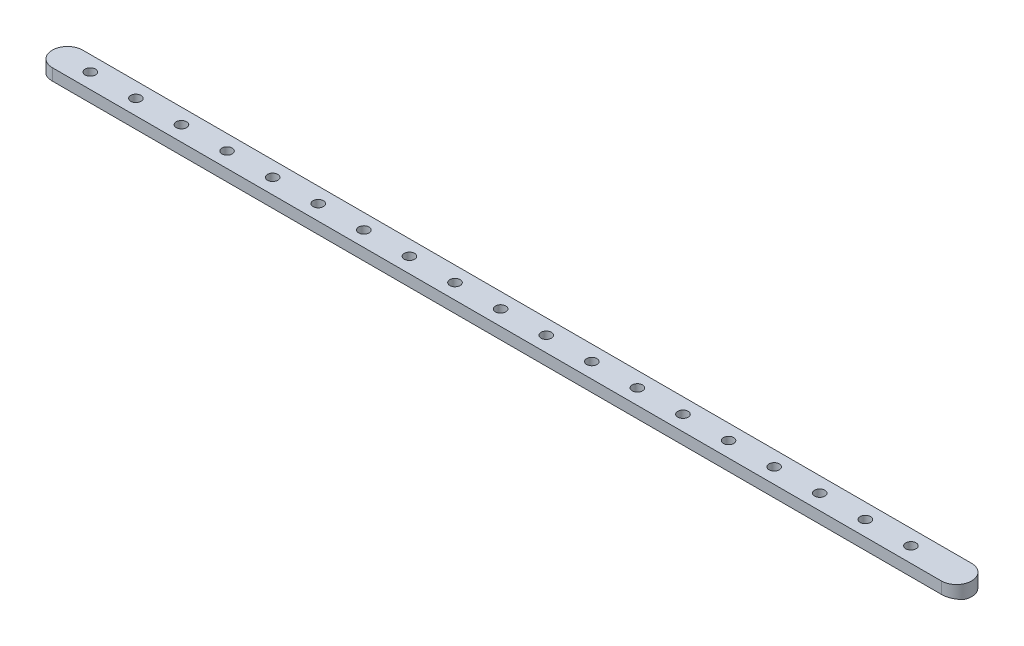
from build123d import *

# Parameters (mm, degrees)
BOSS_EXTRUDE1_DEPTH = 9
M8_TAPPED_HOLE1_D   = 6.8
LPATTERN1_COUNT     = 19
LPATTERN1_PITCH     = 30
CUT_EXTRUDE1_START  = -200
CUT_EXTRUDE1_DEPTH  = 705.20277905


with BuildPart() as part:
    # Sketch1 → Boss-Extrude1 (new body)
    with BuildSketch(Plane(origin=(0, 0, 0), x_dir=(1, 0, 0), z_dir=(0, 1, 0))):
        with BuildLine():
            Line((-90.976744186, 10), (494.023255814, 10))
            ThreePointArc((494.023255814, 10), (504.023255814, 0), (494.023255814, -10))
            Line((494.023255814, -10), (-90.976744186, -10))
            ThreePointArc((-90.976744186, -10), (-100.976744186, 0), (-90.976744186, 10))
        make_face()
    extrude(amount=BOSS_EXTRUDE1_DEPTH)

    # M8 Tapped Hole1 (through all)
    with Locations(Plane(origin=(0, 9, 0), x_dir=(1, 0, 0), z_dir=(0, 1, 0))):
        with Locations((-75.976744186, 0)):
            m8_tapped_hole1 = Hole(M8_TAPPED_HOLE1_D / 2)

    # LPattern1: M8 Tapped Hole1 ×19
    with Locations(*[(i * LPATTERN1_PITCH, 0, 0) for i in range(1, LPATTERN1_COUNT)]):
        add(m8_tapped_hole1, mode=Mode.SUBTRACT)

    # Sketch4 → Cut-Extrude1 (cut, through all)
    with BuildSketch(Plane(origin=(0, 0, 0), x_dir=(0, 0, -1), z_dir=(1, 0, 0)).offset(CUT_EXTRUDE1_START)):
        Polygon((4, 0), (14, 0), (14, 2.216946626), align=None)
        Polygon((-14, 2.216946626), (-14, 0), (-4, 0), align=None)
    extrude(amount=CUT_EXTRUDE1_DEPTH, mode=Mode.SUBTRACT)


solid = part.part
